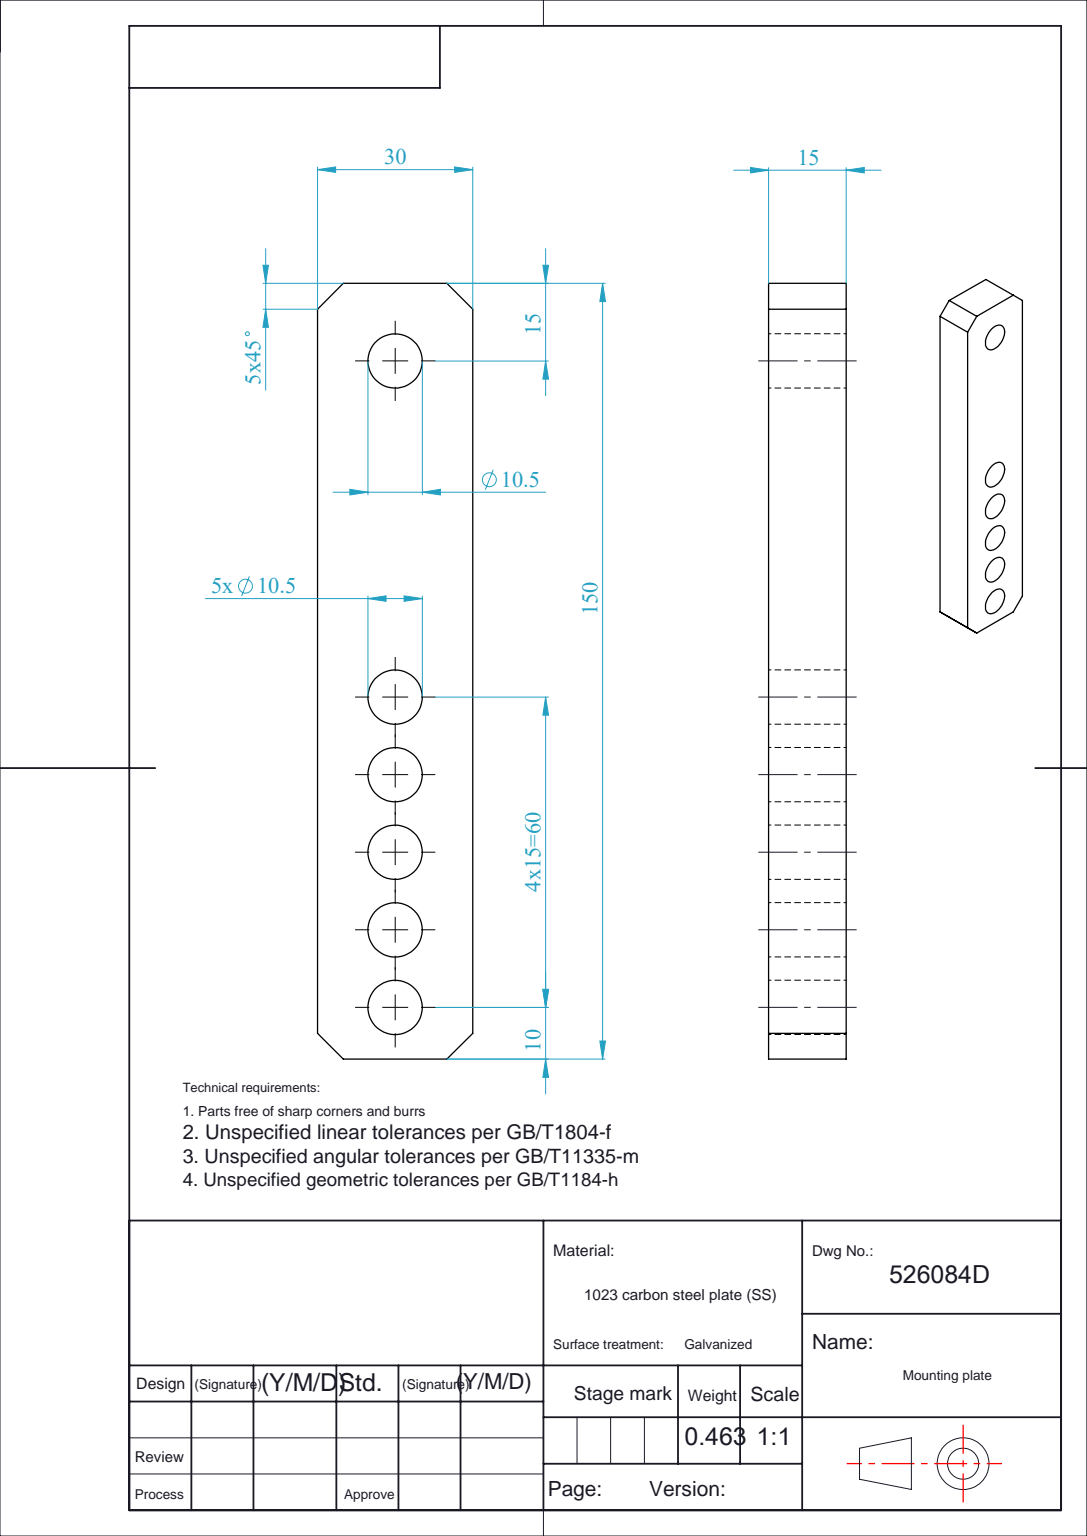
SolidWorks part; units mm, degrees
material "1023 碳钢板 (SS)"
ref_plane "Front Plane" through (0, 0, 0) normal (0, 0, 1) x (1, 0, 0)
ref_plane "Top Plane" through (0, 0, 0) normal (0, 1, 0) x (1, 0, 0)
ref_plane "Right Plane" through (0, 0, 0) normal (1, 0, 0) x (0, 0, -1)
sketch "Sketch1" plane through (0, 0, 0) normal (0, 0, 1) x (1, 0, 0)
  line L1 (-15, 75) -> (15, 75)
  line L2 (-15, 75) -> (-15, -75)
  line L3 (-15, -75) -> (15, -75)
  line L4 (15, 75) -> (15, -75)
  line L5 (-15, 75) -> (15, -75) construction
  line L6 (-15, -75) -> (15, 75) construction
  point P0 (0, 0)
  dimension "D1" = 150
  dimension "D2" = 30
extrude "Boss-Extrude1" add sketch "Sketch1" along normal blind 15
chamfer "Chamfer1" distance 5 angle 45 4 edges at (-15, -75, 7.5) (15, -75, 7.5) (-15, 75, 7.5) (15, 75, 7.5)
sketch "Sketch2" plane through (0, 0, 15) normal (0, 0, 1) x (1, 0, 0)
  line L0 (-10, -75) -> (10, -75) construction
  line L1 (10, 75) -> (-10, 75) construction
  circle A0 centre (0, 60) radius 5.25
  circle A1 centre (0, -5) radius 5.25
  circle A2 centre (0, -20) radius 5.25
  circle A3 centre (0, -35) radius 5.25
  circle A4 centre (0, -50) radius 5.25
  circle A5 centre (0, -65) radius 5.25
  dimension "D1" = 10.5
  dimension "D2" = 15
  dimension "D3" = 15
  dimension "D4" = 15
  dimension "D5" = 25
  dimension "D6" = 15
extrude "Cut-Extrude1" cut sketch "Sketch2" against normal blind 43
